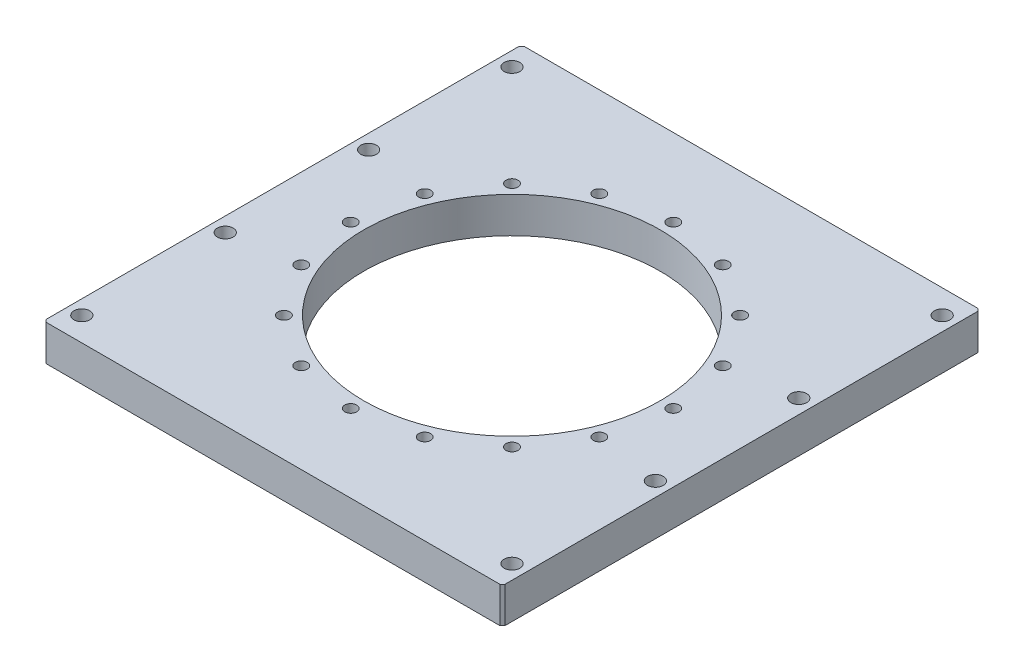
SolidWorks part; units mm, degrees
material "A6061"
ref_plane "前基準面" through (0, 0, 0) normal (0, 0, 1) x (1, 0, 0)
ref_plane "上基準面" through (0, 0, 0) normal (0, 1, 0) x (1, 0, 0)
ref_plane "右基準面" through (0, 0, 0) normal (1, 0, 0) x (0, 0, -1)
sketch "草图1" plane through (0, 0, 0) normal (0, 1, 0) x (1, 0, 0)
  line L1 (-96, -100) -> (96, -100)
  line L2 (-96, -100) -> (-96, 100)
  line L3 (-96, 100) -> (96, 100)
  line L4 (96, -100) -> (96, 100)
  line L5 (-96, -100) -> (96, 100) construction
  line L6 (-96, 100) -> (96, -100) construction
  point P0 (0, 0)
  dimension "D1" = 192
  dimension "D2" = 200
extrude "凸台-拉伸1" add sketch "草图1" along normal mid plane 15
chamfer "倒角1" distance 1 angle 45 4 edges at (96, 0, -100) (96, 0, 100) (-96, 0, -100) (-96, 0, 100)
sketch "草图2" plane through (0, 7.5, 0) normal (0, 1, 0) x (1, 0, 0)
  line L0 (95, 100) -> (-95, 100) construction
  line L1 (-31, -60) -> (31, -60)
  line L2 (-31, -60) -> (-31, 60)
  line L3 (-31, 60) -> (31, 60)
  line L4 (31, -60) -> (31, 60)
  line L5 (-31, -60) -> (31, 60) construction
  line L6 (-31, 60) -> (31, -60) construction
  line L7 (-96, 99) -> (-96, -99) construction
  point P0 (0, 0)
  dimension "D1" = 40
  dimension "D2" = 65
hole_wizard "打孔尺寸(%根据)内六角圆柱头螺钉的类型1" positions "草图6" profile "草图5" counterbore size "M6" standard "GB" end condition through all
sketch "草图6" plane through (0, -7.5, 0) normal (0, -1, 0) x (-1, 0, 0)
  line L0 (0, -123.3943) -> (0, 0) construction
  line L1 (0, 0) -> (142.787, 0) construction
  point P0 (90, -90)
  point P2 (90, -30)
  point P12 (-90, -30)
  point P13 (-90, -90)
  point P14 (-90, 90)
  point P15 (-90, 30)
  point P16 (90, 30)
  point P17 (90, 90)
sketch "草图5" plane through (-90, -7.5, 90) normal (1, 0, 0) x (0, 0, -1)
  line L0 (0, 0) -> (0, 15)
  line L1 (0, 15) -> (3.3, 15)
  line L3 (3.3, 15) -> (3.3, 6.8)
  line L4 (3.3, 6.8) -> (5.5, 6.8)
  line L5 (5.5, 6.8) -> (5.5, 0)
  line L7 (5.5, 0) -> (0, 0)
  line L11 (0, -6.35) -> (0, 107.95) construction
  dimension "通孔孔直径" = 6.6
  dimension "通孔孔深度" = 15
  dimension "柱形沉头孔直径" = 11
  dimension "柱形沉头孔深度" = 6.8
sketch "草图7" plane through (0, 7.5, 0) normal (0, 1, 0) x (1, 0, 0)
  circle A0 centre (0, 0) radius 62
  dimension "D1" = 124
extrude "切除-拉伸1" cut sketch "草图7" against normal up to surface (15 mm away) contours A0 up to face at (-90, -7.5, 84.5)
sketch "草图8" plane through (0, 7.5, 0) normal (0, 1, 0) x (1, 0, 0)
  line L0 (0, 66) -> (0, 100) construction
  line L2 (-37.5, 66) -> (-37.5, 100)
  line L3 (37.5, 66) -> (37.5, 100)
  line L4 (95, 100) -> (-95, 100) construction
  arc A0 (-37.5, 66) -> (37.5, 66) centre (0, 66) ccw
  arc A1 (37.5, 100) -> (-37.5, 100) centre (0, 100) ccw
  circle A3 centre (0, 0) radius 62 construction
  point P5 (0, 83)
  dimension "D1" = 66
  dimension "D2" = 75
hole_wizard "M6 螺纹孔1" positions "草图9" profile "草图10" tap size "M6" standard "GB" end condition through all
sketch "草图9" plane through (0, -7.5, 0) normal (0, -1, 0) x (-1, 0, 0)
  circle A0 centre (0, 0) radius 67.5 construction
  point P27 (67.5, 0)
  point P39 (62.3619, -25.8311)
  point P40 (47.7297, -47.7297)
  point P41 (25.8311, -62.3619)
  point P42 (0, -67.5)
  point P43 (-25.8311, -62.3619)
  point P44 (-47.7297, -47.7297)
  point P45 (-62.3619, -25.8311)
  point P46 (-67.5, 0)
  point P47 (-62.3619, 25.8311)
  point P48 (-47.7297, 47.7297)
  point P49 (-25.8311, 62.3619)
  point P50 (0, 67.5)
  point P51 (25.8311, 62.3619)
  point P52 (47.7297, 47.7297)
  point P53 (62.3619, 25.8311)
  dimension "D2" = 16
  dimension "D1" = 135
sketch "草图10" plane through (-67.5, -7.5, 0) normal (1, 0, 0) x (0, 0, -1)
  line L0 (0, 0) -> (0, 15)
  line L1 (0, 15) -> (2.5, 15)
  line L2 (2.5, 15) -> (2.5, 0)
  line L5 (2.5, 0) -> (0, 0)
  line L11 (0, -6.35) -> (0, 107.95) construction
  dimension "通孔螺纹孔钻头直径" = 5
  dimension "通孔螺纹孔钻头深度" = 15
cosmetic thread "孔螺蚊线1" parameters "D2"=7.6
cosmetic thread "孔螺蚊线2" parameters "D2"=7.6
cosmetic thread "孔螺蚊线3" parameters "D2"=7.6
cosmetic thread "孔螺蚊线4" parameters "D2"=7.6
cosmetic thread "孔螺蚊线5" parameters "D2"=6
cosmetic thread "孔螺蚊线6" parameters "D2"=6
cosmetic thread "孔螺蚊线7" parameters "D2"=6
cosmetic thread "孔螺蚊线8" parameters "D2"=6
cosmetic thread "孔螺蚊线9" parameters "D2"=6
cosmetic thread "孔螺蚊线10" parameters "D2"=6
cosmetic thread "孔螺蚊线11" parameters "D2"=6
cosmetic thread "孔螺蚊线12" parameters "D2"=6
cosmetic thread "孔螺蚊线13" parameters "D2"=6
cosmetic thread "孔螺蚊线14" parameters "D2"=6
cosmetic thread "孔螺蚊线15" parameters "D2"=6
cosmetic thread "孔螺蚊线16" parameters "D2"=6
equation "\"D3@草图6\"=\"D2@草图6\""
